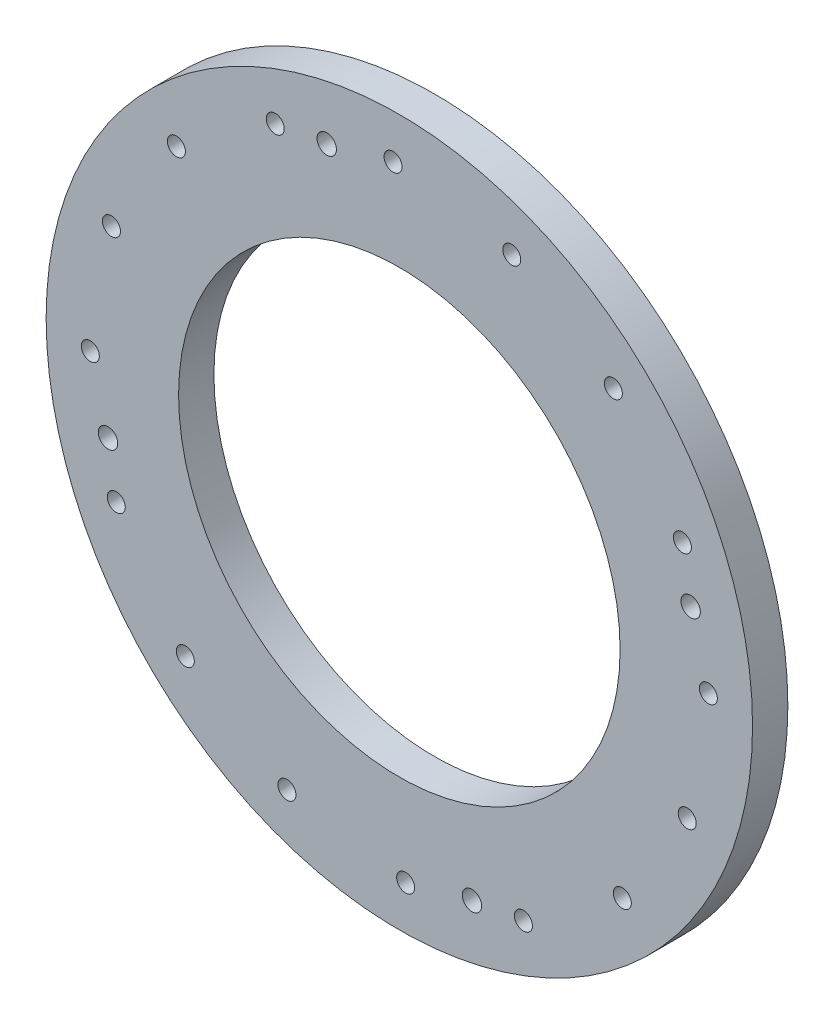
SolidWorks part; units mm, degrees
ref_plane "前视基准面" through (0, 0, 0) normal (0, 0, 1) x (1, 0, 0)
ref_plane "上视基准面" through (0, 0, 0) normal (0, 1, 0) x (1, 0, 0)
ref_plane "右视基准面" through (0, 0, 0) normal (1, 0, 0) x (0, 0, -1)
sketch "草图1" plane through (0, 0, 0) normal (0, 0, 1) x (1, 0, 0)
  circle A0 centre (0, 0) radius 200
  dimension "D1" = 400
extrude "凸台-拉伸1" add sketch "草图1" along normal mid plane 20
sketch "草图2" plane through (0, 0, -10) normal (0, 0, -1) x (-1, 0, 0)
  circle A0 centre (0, 0) radius 125
  dimension "D1" = 250
extrude "切除-拉伸1" cut sketch "草图2" against normal through all
hole_wizard "M12 螺纹孔1" positions "草图4" profile "草图3" tap size "M12" standard "GB" end condition through all
sketch "草图4" plane through (0, 0, -10) normal (0, 0, -1) x (-1, 0, 0)
  circle A0 centre (126.2473, 121.1884) radius 7 construction
  point P1 (126.2473, 121.1884)
sketch "草图3" plane through (-126.2473, 121.1884, -10) normal (1, 0, 0) x (0, 1, 0)
  line L0 (0, 0) -> (0, 20)
  line L1 (0, 20) -> (5.1, 20)
  line L2 (5.1, 20) -> (5.1, 0)
  line L5 (5.1, 0) -> (0, 0)
  line L11 (0, -6.35) -> (0, 107.95) construction
  dimension "通孔螺纹孔钻头直径" = 10.2
  dimension "通孔螺纹孔钻头深度" = 20
cosmetic thread "孔螺蚊线1" parameters "D2"=12
pattern_circular "阵列(圆周)1" count 16 over 360 about axis through (0, 0, 0) along (0, 0, 1) of "M12 螺纹孔1"
hole_wizard "打孔尺寸(%根据)内六角圆柱头螺钉的类型1" positions "草图5" profile "草图6" counterbore size "M10" standard "GB" end condition through all
sketch "草图5" plane through (0, 0, -10) normal (0, 0, -1) x (-1, 0, 0)
  line L0 (0, 0) -> (-164.9503, 41.1267) construction
  line L2 (0, 0) -> (0, 125) construction
  circle A0 centre (0, 0) radius 125 construction
  point P0 (-164.9503, 41.1267)
  dimension "D1" = 170
  dimension "D2" = 76
sketch "草图6" plane through (164.9503, 41.1267, -10) normal (1, 0, 0) x (0, 1, 0)
  line L0 (0, 0) -> (0, 20)
  line L1 (0, 20) -> (5.5, 20)
  line L3 (5.5, 20) -> (5.5, 11)
  line L4 (5.5, 11) -> (9, 11)
  line L5 (9, 11) -> (9, 0)
  line L7 (9, 0) -> (0, 0)
  line L11 (0, -6.35) -> (0, 107.95) construction
  dimension "通孔孔直径" = 11
  dimension "通孔孔深度" = 20
  dimension "柱形沉头孔直径" = 18
  dimension "柱形沉头孔深度" = 11
pattern_circular "阵列(圆周)2" count 4 over 360 about axis through (0, 0, 0) along (0, 0, 1) of "打孔尺寸(%根据)内六角圆柱头螺钉的类型1"
